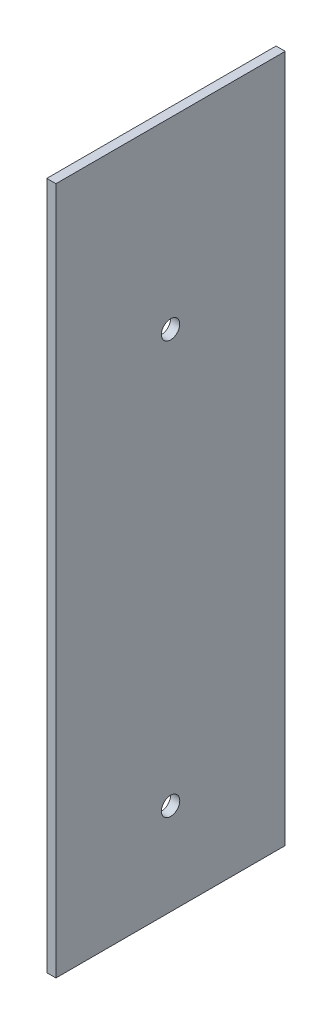
SolidWorks part; units mm, degrees
ref_plane "前视基准面" through (0, 0, 0) normal (0, 0, 1) x (1, 0, 0)
ref_plane "上视基准面" through (0, 0, 0) normal (0, 1, 0) x (1, 0, 0)
ref_plane "右视基准面" through (0, 0, 0) normal (1, 0, 0) x (0, 0, -1)
sketch "草图1" plane through (0, 0, 0) normal (0, 0, 1) x (1, 0, 0)
  line L1 (-1, -90) -> (1, -90)
  line L2 (-1, -90) -> (-1, 90)
  line L3 (-1, 90) -> (1, 90)
  line L4 (1, -90) -> (1, 90)
  line L5 (-1, -90) -> (1, 90) construction
  line L6 (-1, 90) -> (1, -90) construction
  point P0 (0, 0)
  dimension "D1" = 180
  dimension "D2" = 2
extrude "凸台-拉伸1" add sketch "草图1" along normal blind 50
sketch "草图2" plane through (1, 0, 0) normal (1, 0, 0) x (0, 0, -1)
  line L0 (-50, -90) -> (0, -90) construction
  line L1 (0, -90) -> (0, 90) construction
  circle A0 centre (-25, -40) radius 2
  dimension "D1" = 4
  dimension "D2" = 50
  dimension "D3" = 25
extrude "切除-拉伸1" cut sketch "草图2" against normal blind 20
ref_plane "基准面1" through (0, 0, 25) normal (0, 0, 1) x (1, 0, 0)
sketch "草图3" plane through (1, 0, 0) normal (1, 0, 0) x (0, 0, -1)
  line L0 (-25, 1.1) -> (-25, -1.1) construction
  line L1 (-50, 90) -> (0, 90) construction
  circle A0 centre (-25, 50) radius 2
  dimension "D1" = 4
  dimension "D2" = 40
extrude "切除-拉伸2" cut sketch "草图3" against normal blind 10
sketch "草图4" plane through (-1, 0, 0) normal (-1, 0, 0) x (0, 0, 1)
  line L0 (50, -90) -> (0, -90) construction
  line L1 (151.5332, -145.1744) -> (-38.4713, -145.1744)
  line L2 (151.5332, -145.1744) -> (151.5332, -60)
  line L3 (151.5332, -60) -> (-38.4713, -60)
  line L4 (-38.4713, -145.1744) -> (-38.4713, -60)
  line L5 (151.5332, -145.1744) -> (-38.4713, -60) construction
  line L6 (151.5332, -60) -> (-38.4713, -145.1744) construction
  point P0 (56.5309, -102.5872)
  dimension "D1" = 30
extrude "切除-拉伸3" cut sketch "草图4" against normal blind 10
